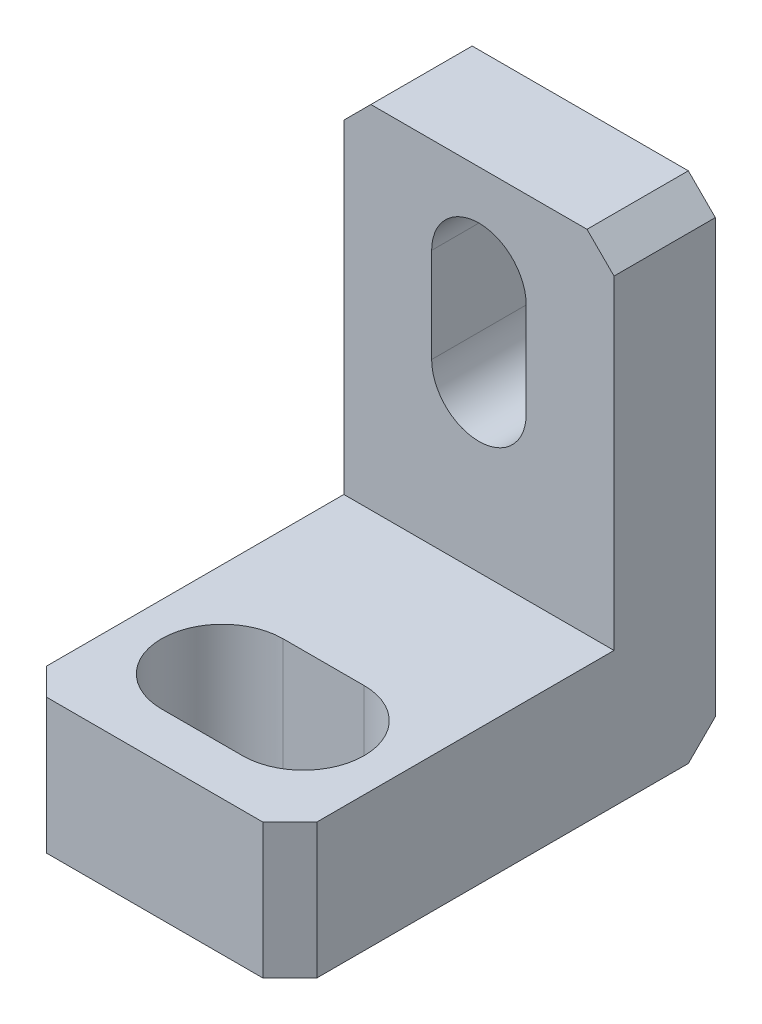
from build123d import *

# Parameters (mm, degrees)
SKETCH1_W           = 10
SKETCH1_H           = 3.75
BOSS_EXTRUDE1_DEPTH = 18
SKETCH2_R           = 1.75
CUT_EXTRUDE1_DEPTH  = 20
SKETCH3_W           = 10
SKETCH3_H           = 12
BOSS_EXTRUDE2_DEPTH = 5
CUT_EXTRUDE2_DEPTH  = 10
CHAMFER1_SIZE       = 1
CUT_EXTRUDE3_DEPTH  = 10


with BuildPart() as part:
    # Sketch1 → Boss-Extrude1 (new body)
    with BuildSketch(Plane(origin=(0, 0, 0), x_dir=(1, 0, 0), z_dir=(0, 1, 0))):
        with Locations((5, 1.875)):
            Rectangle(SKETCH1_W, SKETCH1_H)
    extrude(amount=BOSS_EXTRUDE1_DEPTH)

    # Sketch2 → Cut-Extrude1 (cut)
    with BuildSketch(Plane.XY):
        with Locations((5, 12.7)):
            Circle(SKETCH2_R)
    extrude(amount=-CUT_EXTRUDE1_DEPTH, mode=Mode.SUBTRACT)

    # Sketch3 → Boss-Extrude2 (add)
    with BuildSketch(Plane.XZ):
        with Locations((5, 6)):
            Rectangle(SKETCH3_W, SKETCH3_H)
    extrude(amount=-BOSS_EXTRUDE2_DEPTH)

    # Sketch4 → Cut-Extrude2 (cut)
    with BuildSketch(Plane(origin=(0, 5, 0), x_dir=(1, 0, 0), z_dir=(0, 1, 0))):
        with BuildLine():
            Line((3.5, -10.25), (6.5, -10.25))
            ThreePointArc((6.5, -10.25), (8.75, -8), (6.5, -5.75))
            Line((6.5, -5.75), (3.5, -5.75))
            ThreePointArc((3.5, -5.75), (1.25, -8), (3.5, -10.25))
        make_face()
    extrude(amount=-CUT_EXTRUDE2_DEPTH, mode=Mode.SUBTRACT)

    # Chamfer1
    chamfer1_edges = [part.edges().sort_by_distance(p)[0] for p in [
        (10, 18, -1.875),
        (0, 2.5, 12),
        (10, 2.5, 12),
        (0, 18, -1.875),
        (5, 0, -3.75),
    ]]
    chamfer(chamfer1_edges, length=CHAMFER1_SIZE)

    # Sketch5 → Cut-Extrude3 (cut)
    with BuildSketch(Plane.XY):
        with BuildLine():
            Line((6.75, 14.45), (6.75, 10.95))
            ThreePointArc((6.75, 10.95), (5, 9.2), (3.25, 10.95))
            Line((3.25, 10.95), (3.25, 14.45))
            ThreePointArc((3.25, 14.45), (5, 16.2), (6.75, 14.45))
        make_face()
    extrude(amount=-CUT_EXTRUDE3_DEPTH, mode=Mode.SUBTRACT)


solid = part.part
